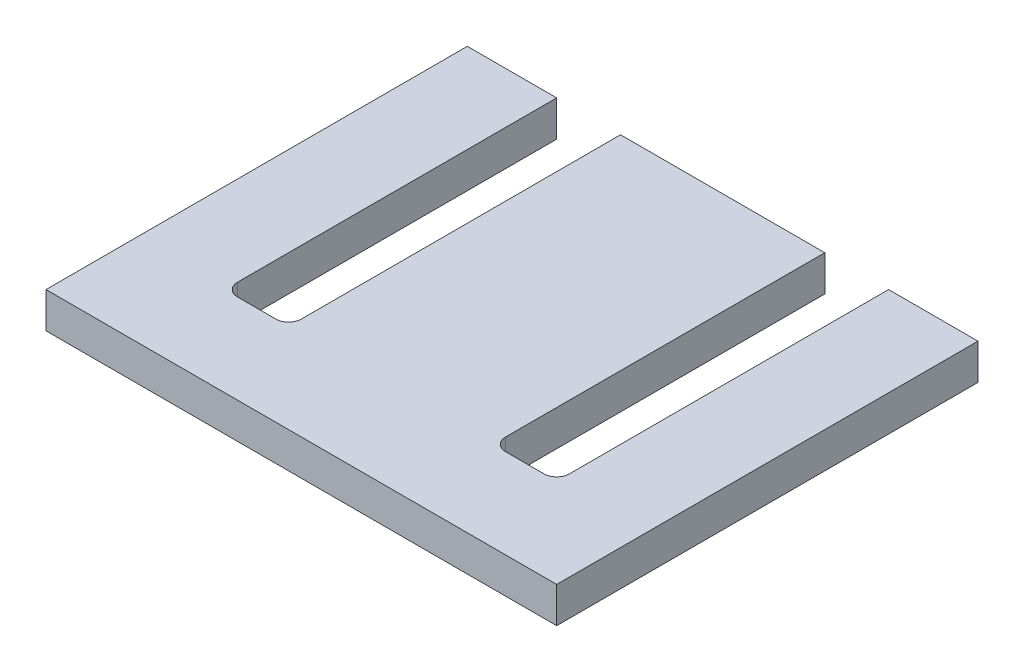
from build123d import *

# Parameters (mm, degrees)
SKETCH_1_W          = 200
SKETCH_1_H          = 165
EXTRUDE_1_DEPTH     = 14
CUT_EXTRUDE_1_REACH = 132.393
SKETCH_2_W          = 25
SKETCH_2_H          = 130
FILLET_1_R          = 5


with BuildPart() as part:
    # 草图1 → 凸台-拉伸1 (new body)
    with BuildSketch(Plane(origin=(0, 0, 0), x_dir=(1, 0, 0), z_dir=(0, 1, 0))):
        Rectangle(SKETCH_1_W, SKETCH_1_H)
    extrude(amount=EXTRUDE_1_DEPTH)

    # 草图2 → 切除-拉伸1 (cut, up to next)
    with BuildSketch(Plane.XZ, mode=Mode.PRIVATE) as cut_extrude_1_sk1:
        with Locations((52.5, -17.5)):
            Rectangle(SKETCH_2_W, SKETCH_2_H)
    cut_extrude_1_tool1 = extrude(cut_extrude_1_sk1.sketch, amount=-CUT_EXTRUDE_1_REACH, mode=Mode.PRIVATE) & part.part
    # 草图2 → 切除-拉伸1 (cut, up to next)
    with BuildSketch(Plane.XZ, mode=Mode.PRIVATE) as cut_extrude_1_sk2:
        with Locations((-52.5, -17.5)):
            Rectangle(SKETCH_2_W, SKETCH_2_H)
    cut_extrude_1_tool2 = extrude(cut_extrude_1_sk2.sketch, amount=-CUT_EXTRUDE_1_REACH, mode=Mode.PRIVATE) & part.part
    add(cut_extrude_1_tool1.solids().sort_by_distance((52.5, 0, -17.5))[0], mode=Mode.SUBTRACT)
    add(cut_extrude_1_tool2.solids().sort_by_distance((-52.5, 0, -17.5))[0], mode=Mode.SUBTRACT)

    # 圆角1
    fillet_1_edges = [part.edges().sort_by_distance(p)[0] for p in [
        (40, 7, 47.5),
        (65, 7, 47.5),
        (-40, 7, 47.5),
        (-65, 7, 47.5),
    ]]
    fillet(fillet_1_edges, radius=FILLET_1_R)


solid = part.part
